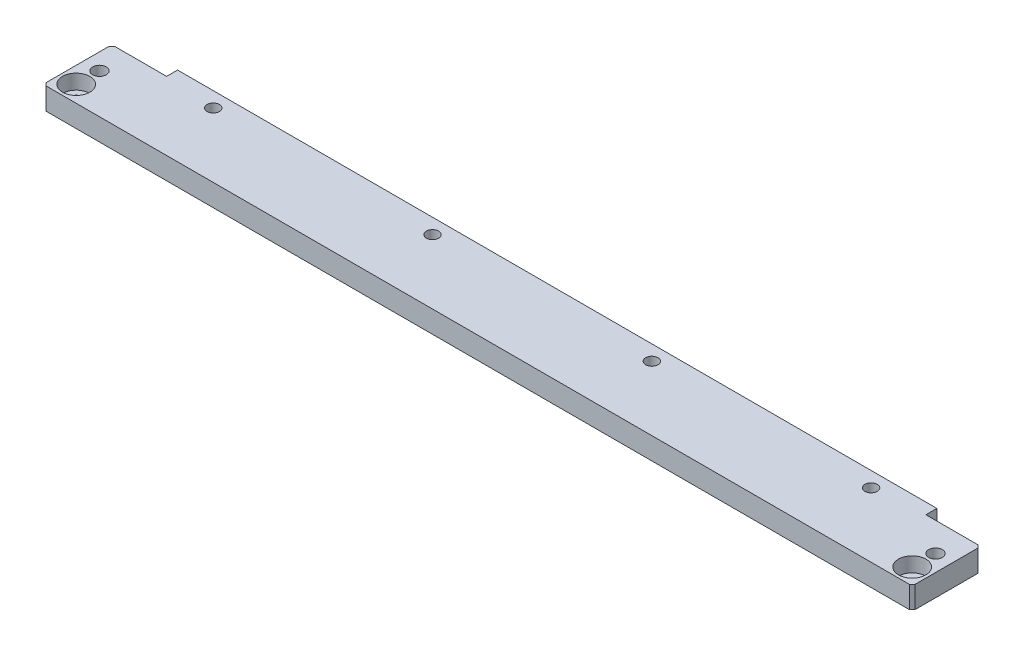
SolidWorks part; units mm, degrees
material "Al6061"
ref_plane "Front" through (0, 0, 0) normal (0, 0, 1) x (1, 0, 0)
ref_plane "Top" through (0, 0, 0) normal (0, 1, 0) x (1, 0, 0)
ref_plane "Right" through (0, 0, 0) normal (1, 0, 0) x (0, 0, -1)
sketch "草图1" plane through (0, 0, 0) normal (0, 1, 0) x (1, 0, 0)
  line L1 (-158.5, 12.5) -> (158.5, 12.5)
  line L2 (-158.5, 12.5) -> (-158.5, -12.5)
  line L3 (-158.5, -12.5) -> (158.5, -12.5)
  line L4 (158.5, 12.5) -> (158.5, -12.5)
  line L5 (-158.5, 12.5) -> (158.5, -12.5) construction
  line L6 (-158.5, -12.5) -> (158.5, 12.5) construction
  point P0 (0, 0)
  dimension "D1" = 25
  dimension "D2" = 317
extrude "凸台-拉伸1" add sketch "草图1" along normal blind 8
hole_wizard "M5 六角凹头螺钉的柱形沉头孔1" positions "草图3" profile "草图2" counterbore size "M5" standard "Iso" end condition through all
sketch "草图3" plane through (0, 8, 0) normal (0, 1, 0) x (1, 0, 0)
  line L0 (-158.5, 12.5) -> (-158.5, -12.5) construction
  line L1 (-158.5, -12.5) -> (158.5, -12.5) construction
  line L2 (158.5, -12.5) -> (158.5, 12.5) construction
  point P0 (-152.5, -6.5)
  point P2 (152.5, -6.5)
  dimension "D1" = 6
  dimension "D2" = 6
  dimension "D3" = 6
sketch "草图2" plane through (-152.5, 8, 6.5) normal (1, 0, 0) x (0, 0, 1)
  line L0 (0, 0) -> (0, 8)
  line L1 (0, 8) -> (2.75, 8)
  line L3 (2.75, 8) -> (2.75, 5.4)
  line L4 (2.75, 5.4) -> (5, 5.4)
  line L5 (5, 5.4) -> (5, 0)
  line L7 (5, 0) -> (0, 0)
  line L11 (0, -6.35) -> (0, 107.95) construction
  dimension "通孔孔直径" = 5.5
  dimension "通孔孔深度" = 8
  dimension "柱形沉头孔直径" = 10
  dimension "柱形沉头孔深度" = 5.4
sketch "草图4" plane through (0, 8, 0) normal (0, 1, 0) x (1, 0, 0)
  line L0 (-158.5, 2) -> (158.5, 2) construction
  line L1 (-158.5, 12.5) -> (-158.5, -12.5) construction
  line L2 (158.5, -12.5) -> (158.5, 12.5) construction
  line L3 (-152.5, -6.5) -> (-152.5, 2) construction
  line L4 (152.5, -6.5) -> (152.5, 2) construction
  circle A0 centre (-152.5, 2) radius 2.5
  circle A1 centre (152.5, 2) radius 2.5
  circle A2 centre (152.5, -6.5) radius 5 construction
  dimension "D1" = 5
  dimension "D2" = 8.5
extrude "切除-拉伸1" cut sketch "草图4" against normal through all
sketch "草图7" plane through (0, 0, 0) normal (0, -1, 0) x (1, 0, 0)
  line L0 (158.5, -12.5) -> (-158.5, -12.5) construction
  line L1 (-138.5, -12.5) -> (138.5, -12.5)
  line L2 (-138.5, -12.5) -> (-138.5, -16.5)
  line L3 (-138.5, -16.5) -> (138.5, -16.5)
  line L4 (138.5, -12.5) -> (138.5, -16.5)
  line L5 (0, 0) -> (0, -12.5) construction
  dimension "D1" = 4
  dimension "D2" = 277
extrude "凸台-拉伸2" add sketch "草图7" against normal up to surface (8 mm away) up to face at (152.5, 8, 0.5)
hole_wizard "M4 六角凹头螺钉的柱形沉头孔1" positions "草图6" profile "草图5" counterbore size "M4" standard "Iso" end condition through all
sketch "草图6" plane through (0, 0, 0) normal (0, -1, 0) x (-1, 0, 0)
  line L0 (0, 0) -> (0, 16.5) construction
  line L3 (138.5, 16.5) -> (-138.5, 16.5) construction
  point P0 (-120, 11)
  point P2 (-40, 11)
  point P4 (40, 11)
  point P6 (120, 11)
  dimension "D1" = 5.5
  dimension "D2" = 80
  dimension "D3" = 80
sketch "草图5" plane through (120, 0, -11) normal (1, 0, 0) x (0, 0, -1)
  line L0 (0, 0) -> (0, 8.0001)
  line L1 (0, 8.0001) -> (2.25, 8.0001)
  line L3 (2.25, 8.0001) -> (2.25, 4.4)
  line L4 (2.25, 4.4) -> (4, 4.4)
  line L5 (4, 4.4) -> (4, 0)
  line L7 (4, 0) -> (0, 0)
  line L11 (0, -6.35) -> (0, 107.95) construction
  dimension "通孔孔直径" = 4.5
  dimension "通孔孔深度" = 8.0001
  dimension "柱形沉头孔直径" = 8
  dimension "柱形沉头孔深度" = 4.4
chamfer "倒角3" distance 1 angle 45 4 edges at (-158.5, 4, -12.5) (-158.5, 4, 12.5) (158.5, 4, -12.5) (158.5, 4, 12.5)
